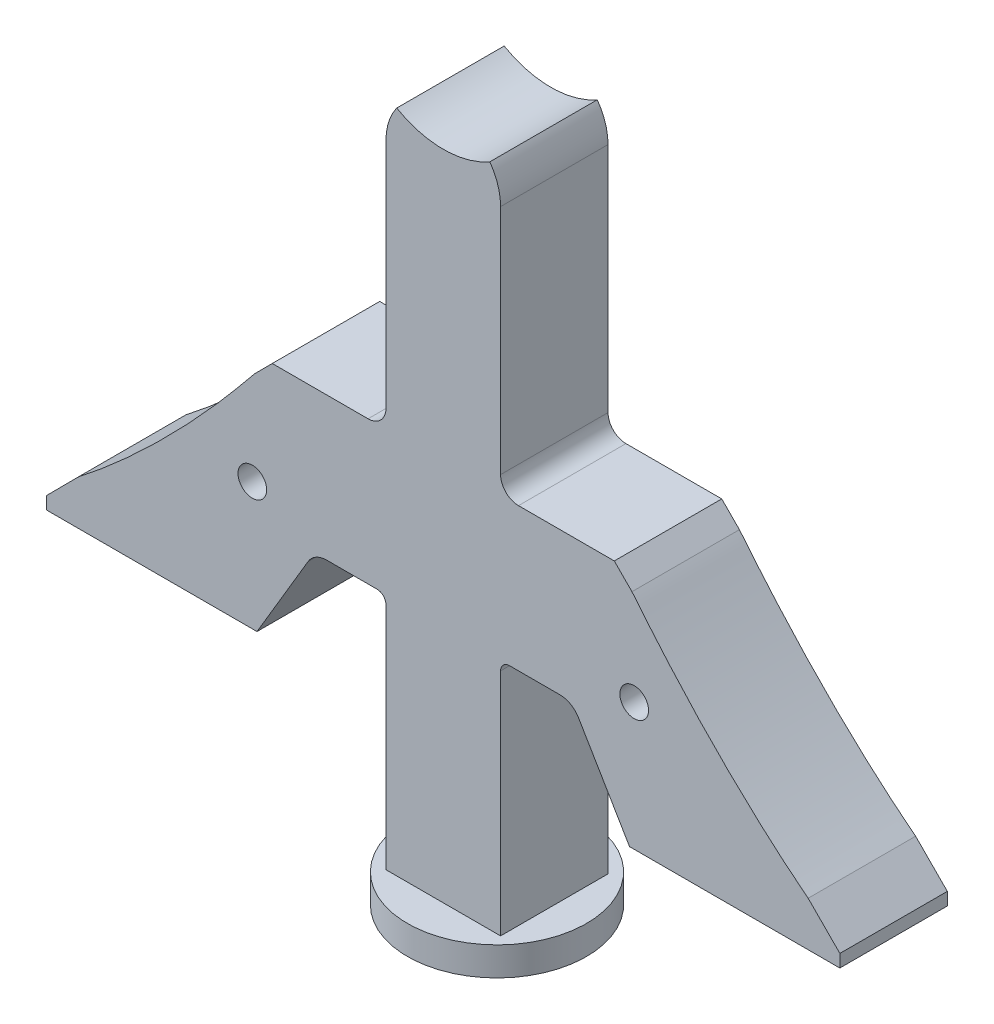
from build123d import *
from OCP.BRepFilletAPI import BRepFilletAPI_MakeChamfer

# Parameters (mm, degrees)
BOSS_EXTRUDE1_DEPTH      = 10
BOSS_EXTRUDE2_DEPTH      = 10
SKETCH72_R               = 5
CUT_EXTRUDE2_DEPTH       = 10
CUT_EXTRUDE4_DEPTH       = 14
CUT_EXTRUDE4_DEPTH_BACK  = 19
BOSS_EXTRUDE3_START      = 20
BOSS_EXTRUDE3_DEPTH      = 20
CUT_EXTRUDE5_DEPTH       = 19
CUT_EXTRUDE5_DEPTH_BACK  = 48
SKETCH146_R              = 5
CUT_EXTRUDE6_DEPTH       = 19
CUT_EXTRUDE6_DEPTH_BACK  = 19
CUT_EXTRUDE7_DEPTH       = 60
CUT_EXTRUDE8_DEPTH       = 72
CUT_EXTRUDE9_DEPTH       = 88
BOSS_EXTRUDE6_START      = -7.5
BOSS_EXTRUDE6_DEPTH      = 7.5
CUT_EXTRUDE10_DEPTH      = 19
CUT_EXTRUDE10_DEPTH_BACK = 41
SKETCH171_R              = 5
BOSS_EXTRUDE7_DEPTH      = 7.5
SKETCH172_W              = 3
SKETCH172_H              = 35.030253814
BOSS_EXTRUDE8_DEPTH      = 15
SKETCH173_W              = 32
SKETCH173_H              = 200
BOSS_EXTRUDE9_DEPTH      = 30
CHAMFER1_SIZE            = 5
CHAMFER1_SIZE2           = 3.535553346
FILLET1_R                = 5
CUT_EXTRUDE11_DEPTH      = 30
SKETCH175_W              = 47.76869264
SKETCH175_H              = 185.151923251
CUT_EXTRUDE12_DEPTH      = 55
SKETCH151_R              = 4
CUT_EXTRUDE14_DEPTH      = 15
SKETCH153_R              = 4
CUT_EXTRUDE15_DEPTH      = 15
CHAMFER3_SIZE            = 0.5
BOSS_EXTRUDE10_DEPTH     = 30
CUT_EXTRUDE16_DEPTH      = 181.457563316
SKETCH179_R              = 25
BOSS_EXTRUDE11_DEPTH     = 8


with BuildPart() as part:
    # Sketch1 → Boss-Extrude1 (new body)
    with BuildSketch(Plane.XY):
        with BuildLine():
            Line((-15, 37.030253814), (-15, -127.65801455))
            Line((-15, -127.65801455), (15, -127.65801455))
            Line((15, -127.65801455), (15, 37.030253814))
            ThreePointArc((15, 37.030253814), (0, 52.030253814), (-15, 37.030253814))
        make_face()
    extrude(amount=BOSS_EXTRUDE1_DEPTH)

    # Sketch2 → Boss-Extrude2 (add)
    with BuildSketch(Plane(origin=(0, 0, 0), x_dir=(-1, 0, 0), z_dir=(0, 0, -1))):
        Polygon((0, -15), (30.09, -15), (139.247111701, -124.883480474), (-139.247111701, -124.883480474), (-30.09, -15), align=None)
    extrude(amount=-BOSS_EXTRUDE2_DEPTH)

    # Sketch72 → Cut-Extrude2 (cut)
    with BuildSketch(Plane.XY.offset(10)):
        with Locations((0, 37.030253814)):
            Circle(SKETCH72_R)
    extrude(amount=-CUT_EXTRUDE2_DEPTH, mode=Mode.SUBTRACT)

    # Sketch144 → Cut-Extrude4 (cut, two sides: drawn at the far end of the back side and taken through both)
    with BuildSketch(Plane.XY.offset(10).offset(-CUT_EXTRUDE4_DEPTH_BACK)):
        with BuildLine():
            Line((-13, 37.030253814), (-13, -15))
            Line((-13, -15), (-23, -15))
            Line((-23, -15), (-23, 37.030253814))
            ThreePointArc((-23, 37.030253814), (0, 60.030253814), (23, 37.030253814))
            Line((23, 37.030253814), (23, -15))
            Line((23, -15), (13, -15))
            Line((13, -15), (13, 37.030253814))
            ThreePointArc((13, 37.030253814), (0, 50.030253814), (-13, 37.030253814))
        make_face()
    extrude(amount=CUT_EXTRUDE4_DEPTH + CUT_EXTRUDE4_DEPTH_BACK, mode=Mode.SUBTRACT)

    # Sketch145 → Boss-Extrude3 (add)
    with BuildSketch(Plane(origin=(0, 0, 0), x_dir=(-1, 0, 0), z_dir=(0, 0, -1)).offset(BOSS_EXTRUDE3_START)):
        with BuildLine():
            Line((30.09, -15), (13, -15))
            Line((13, -15), (13, 37.030253814))
            ThreePointArc((13, 37.030253814), (0, 50.030253814), (-13, 37.030253814))
            Line((-13, 37.030253814), (-13, -15))
            Line((-13, -15), (-30.09, -15))
            Line((-30.09, -15), (-139.247111701, -124.883480474))
            Line((-139.247111701, -124.883480474), (-15, -124.883480474))
            Line((-15, -124.883480474), (-15, -127.65801455))
            Line((-15, -127.65801455), (15, -127.65801455))
            Line((15, -127.65801455), (15, -124.883480474))
            Line((15, -124.883480474), (139.247111701, -124.883480474))
            Line((139.247111701, -124.883480474), (30.09, -15))
        make_face()
    extrude(amount=-BOSS_EXTRUDE3_DEPTH)

    # Sketch146 → Cut-Extrude5 (cut, two sides: drawn at the far end of the back side and taken through both)
    with BuildSketch(Plane.XY.offset(-CUT_EXTRUDE5_DEPTH_BACK)):
        with Locations((0, 37.030253814)):
            Circle(SKETCH146_R)
    extrude(amount=CUT_EXTRUDE5_DEPTH + CUT_EXTRUDE5_DEPTH_BACK, mode=Mode.SUBTRACT)

    # Sketch147 → Cut-Extrude6 (cut, two sides: drawn at the far end of the back side and taken through both)
    with BuildSketch(Plane(origin=(0, 0, 0), x_dir=(0, 0, -1), z_dir=(1, 0, 0)).offset(-CUT_EXTRUDE6_DEPTH_BACK)):
        Polygon((-2.5, 50.030253814), (-2.5, 20.030253814), (12.5, 20.030253814), (12.5, 50.030253814), (5, 50.030253814), align=None)
    extrude(amount=CUT_EXTRUDE6_DEPTH + CUT_EXTRUDE6_DEPTH_BACK, mode=Mode.SUBTRACT)

    # Sketch150 → Cut-Extrude7 (cut)
    with BuildSketch(Plane.XY.offset(10)):
        Polygon((-139.247111701, -124.883480474), (-114.247111701, -124.883480474), (-114.247111701, -93.838923463), (-155.604312259, -93.838923463), align=None)
        Polygon((139.247111701, -124.883480474), (114.247111701, -124.883480474), (114.247111701, -93.838923463), (144.778818184, -93.838923463), align=None)
    extrude(amount=-CUT_EXTRUDE7_DEPTH, mode=Mode.SUBTRACT)

    # Sketch155 → Cut-Extrude8 (cut)
    with BuildSketch(Plane(origin=(0, 0, -20), x_dir=(-1, 0, 0), z_dir=(0, 0, -1))):
        Polygon((-114.247111701, -99.71712192), (114.247111701, -99.71712192), (132.998124018, -127.280721413), (-4.838954003, -174.810748317), (-128.945135363, -139.691339549), align=None)
    extrude(amount=-CUT_EXTRUDE8_DEPTH, mode=Mode.SUBTRACT)

    # Sketch168 → Cut-Extrude9 (cut)
    with BuildSketch(Plane.XY.offset(10)):
        with BuildLine():
            Line((-102.627965354, -87.973722378), (-98.21134674, -23.838785425))
            Line((-98.21134674, -23.838785425), (-52.676683547, -37.736983068))
            add(Edge.make_bspline(
                [(-52.676683547, -37.736983068), (-53.448253243, -38.604940944), (-54.758018803, -40.255486938), (-56.393307349, -42.24544513), (-57.59393724, -43.693311358), (-58.490883563, -44.765164273), (-59.386563239, -45.826752691), (-60.281018922, -46.878039923), (-61.174144179, -47.919111167), (-62.065873359, -48.950018312), (-62.956131171, -49.970821146), (-63.844846057, -50.981576429), (-64.731946625, -51.982340808), (-65.617362588, -52.973170047), (-66.501024502, -53.954119244), (-67.382863834, -54.925242774), (-68.262812936, -55.886594308), (-69.140805058, -56.83822681), (-70.016774341, -57.78019253), (-70.890655834, -58.712543006), (-71.762385492, -59.635329052), (-72.6319002, -60.548600748), (-73.499137782, -61.452407427), (-74.36403703, -62.346797658), (-75.226537723, -63.231819226), (-76.086580666, -64.107519102), (-76.944107728, -64.97394342), (-77.799061885, -65.83113743), (-78.651387281, -66.679145464), (-79.501029286, -67.518010878), (-80.347934579, -68.347775997), (-81.192051232, -69.16848204), (-82.033328819, -69.980169042), (-82.871718537, -70.782875754), (-83.707173346, -71.576639531), (-84.539648144, -72.3614962), (-85.369099962, -73.137479905), (-86.195488195, -73.90462292), (-87.018774882, -74.662955436), (-87.838925031, -75.412505303), (-88.655907003, -76.153297726), (-89.469692983, -76.885354899), (-90.280259527, -77.608695576), (-91.08758824, -78.323334537), (-91.89166658, -79.029281964), (-92.692488851, -79.726542658), (-93.490057409, -80.415115104), (-94.284384181, -81.094990278), (-95.075492456, -81.766150286), (-95.86341948, -82.428566214), (-96.6482185, -83.08219705), (-97.429965937, -83.726982263), (-98.208753829, -84.362854554), (-98.984742254, -84.989673948), (-99.757998209, -85.607446121), (-100.529132919, -86.215484264), (-101.170253751, -86.716417382), (-101.895413536, -87.270801703), (-102.35237684, -87.641445426), (-102.627965354, -87.973722378)],
                knots=[0, 0, 0, 0, 0.049042517, 0.089027758, 0.108836127, 0.128522053, 0.148085836, 0.167527768, 0.186848129, 0.20604719, 0.225125215, 0.244082454, 0.262919153, 0.281635546, 0.30023186, 0.318708314, 0.337065118, 0.355302476, 0.373420583, 0.391419629, 0.409299796, 0.427061258, 0.444704186, 0.462228743, 0.479635086, 0.496923368, 0.514093738, 0.531146337, 0.548081305, 0.564898777, 0.581598887, 0.598181763, 0.614647534, 0.630996326, 0.647228265, 0.66334348, 0.679342097, 0.695224248, 0.710990068, 0.7266397, 0.742173292, 0.757591004, 0.772893008, 0.788079493, 0.803150668, 0.81810677, 0.832948063, 0.847674856, 0.862287502, 0.876786419, 0.8911721, 0.905445137, 0.919606246, 0.933656302, 0.94759639, 0.961427866, 0.975152458, 0.981975355, 1, 1, 1, 1], degree=3))
        make_face()
    cut_extrude9 = extrude(amount=-CUT_EXTRUDE9_DEPTH, mode=Mode.SUBTRACT)

    # Mirror1: Cut-Extrude9 across plane
    add(cut_extrude9.mirror(Plane(origin=(0, 0, 0), x_dir=(0, 0, 1), z_dir=(1, 0, 0))), mode=Mode.SUBTRACT)

    # Sketch169 → Boss-Extrude6 (add)
    with BuildSketch(Plane.XY.offset(10).offset(BOSS_EXTRUDE6_START)):
        with BuildLine():
            Line((-16, -15), (-13, -15))
            Line((-13, -15), (-13, 37.030253814))
            ThreePointArc((-13, 37.030253814), (-12.375631297, 41.010674647), (-10.5625, 44.608749295))
            Line((-10.5625, 44.608749295), (-16, 37.030253814))
            Line((-16, 37.030253814), (-16, -15))
        make_face()
        with BuildLine():
            Line((16, -15), (16, 37.030253814))
            Line((16, 37.030253814), (10.5625, 44.608749295))
            ThreePointArc((10.5625, 44.608749295), (12.375631297, 41.010674647), (13, 37.030253814))
            Line((13, 37.030253814), (13, -15))
            Line((13, -15), (16, -15))
        make_face()
    extrude(amount=BOSS_EXTRUDE6_DEPTH)

    # Sketch170 → Cut-Extrude10 (cut, two sides: drawn at the far end of the back side and taken through both)
    with BuildSketch(Plane.XY.offset(10).offset(-CUT_EXTRUDE10_DEPTH_BACK)):
        Polygon((-63.887492501, -32.771153319), (-27.188421499, -2.740818682), (-16, -2.740818682), (-16, -15), (-16, -32.771153319), align=None)
        Polygon((16, -15), (16, -32.771153319), (63.887492501, -32.771153319), (27.188421499, -2.740818682), (16, -2.740818682), align=None)
    extrude(amount=CUT_EXTRUDE10_DEPTH + CUT_EXTRUDE10_DEPTH_BACK, mode=Mode.SUBTRACT)

    # Sketch171 → Boss-Extrude7 (add)
    with BuildSketch(Plane(origin=(0, 0, -20), x_dir=(-1, 0, 0), z_dir=(0, 0, -1))):
        with BuildLine():
            Line((16, -15), (-16, -15))
            Line((-16, -15), (-16, 37.030253814))
            Line((-16, 37.030253814), (-10.5625, 44.608749295))
            ThreePointArc((-10.5625, 44.608749295), (0, 50.030253814), (10.5625, 44.608749295))
            Line((10.5625, 44.608749295), (16, 37.030253814))
            Line((16, 37.030253814), (16, -15))
        make_face()
        with Locations(Location((0, 37.030253814, 0), (0, 0, 180))):
            Circle(SKETCH171_R, mode=Mode.SUBTRACT)
    extrude(amount=-BOSS_EXTRUDE7_DEPTH)

    # Sketch172 → Boss-Extrude8 (add)
    with BuildSketch(Plane(origin=(0, 0, 2.5), x_dir=(-1, 0, 0), z_dir=(0, 0, -1))):
        with Locations((-14.5, 2.515126907)):
            Rectangle(SKETCH172_W, SKETCH172_H)
        with Locations((14.5, 2.515126907)):
            Rectangle(SKETCH172_W, SKETCH172_H)
    extrude(amount=BOSS_EXTRUDE8_DEPTH)

    # Sketch173 → Boss-Extrude9 (add)
    with BuildSketch(Plane(origin=(0, 0, -20), x_dir=(-1, 0, 0), z_dir=(0, 0, -1))):
        with Locations((0, -199.71712192)):
            Rectangle(SKETCH173_W, SKETCH173_H)
    extrude(amount=-BOSS_EXTRUDE9_DEPTH)

    # Chamfer1: one chamfer whose edges measure the first distance from different faces: ONE call of the kernel's chamfer builder (chamfer() names one face for all edges)
    chamfer1_edges_1 = [part.edges().sort_by_distance(p)[0] for p in [
        (-114.247111701, -99.71712192, -5),
    ]]
    chamfer1_side_1 = [part.faces().sort_by_distance(p)[0] for p in [
        (-108.057185848, -93.486006182, -5),
    ]]
    chamfer1_edges_2 = [part.edges().sort_by_distance(p)[0] for p in [
        (114.247111701, -99.71712192, -5),
    ]]
    chamfer1_side_2 = [part.faces().sort_by_distance(p)[0] for p in [
        (108.057185848, -93.486006182, -5),
    ]]
    chamfer1 = BRepFilletAPI_MakeChamfer(part.part.solid().wrapped)
    for e in chamfer1_edges_1:
        chamfer1.Add(CHAMFER1_SIZE, CHAMFER1_SIZE2, e.wrapped, chamfer1_side_1[0].wrapped)  # the first distance lies on this face
    for e in chamfer1_edges_2:
        chamfer1.Add(CHAMFER1_SIZE, CHAMFER1_SIZE2, e.wrapped, chamfer1_side_2[0].wrapped)  # the first distance lies on this face
    add(Compound.cast(chamfer1.Shape()), mode=Mode.REPLACE)

    # Fillet1
    fillet1_edges = [part.edges().sort_by_distance(p)[0] for p in [
        (-16, -32.771153319, -5),
        (16, -32.771153319, -5),
    ]]
    fillet(fillet1_edges, radius=FILLET1_R)

    # Sketch174 → Cut-Extrude11 (cut)
    with BuildSketch(Plane.XY.offset(10)):
        with BuildLine():
            Line((-16, -99.71712192), (-16, -75.21712192))
            ThreePointArc((-16, -75.21712192), (-16.732233047, -73.449354967), (-18.5, -72.71712192))
            Line((-18.5, -72.71712192), (-32.581175633, -72.71712192))
            ThreePointArc((-32.581175633, -72.71712192), (-35.551622901, -73.504018907), (-37.742924834, -75.658307578))
            Line((-37.742924834, -75.658307578), (-52, -99.71712192))
            Line((-52, -99.71712192), (-16, -99.71712192))
        make_face()
        with BuildLine():
            Line((16, -99.71712192), (52, -99.71712192))
            Line((52, -99.71712192), (37.742924834, -75.658307578))
            ThreePointArc((37.742924834, -75.658307578), (35.551622901, -73.504018907), (32.581175633, -72.71712192))
            Line((32.581175633, -72.71712192), (18.5, -72.71712192))
            ThreePointArc((18.5, -72.71712192), (16.732233047, -73.449354967), (16, -75.21712192))
            Line((16, -75.21712192), (16, -99.71712192))
        make_face()
    extrude(amount=-CUT_EXTRUDE11_DEPTH, mode=Mode.SUBTRACT)

    # Sketch175 → Cut-Extrude12 (cut)
    with BuildSketch(Plane.XY.offset(10)):
        with Locations((-3.11565368, -231.878790674)):
            Rectangle(SKETCH175_W, SKETCH175_H)
    extrude(amount=-CUT_EXTRUDE12_DEPTH, mode=Mode.SUBTRACT)

    # Sketch151 → Cut-Extrude14 (cut)
    with BuildSketch(Plane.XY.offset(10)):
        with Locations((-53.305086147, -64.131398819)):
            Circle(SKETCH151_R)
    extrude(amount=-CUT_EXTRUDE14_DEPTH, mode=Mode.SUBTRACT)

    # Sketch153 → Cut-Extrude15 (cut)
    with BuildSketch(Plane.XY.offset(10)):
        with Locations(Location((53.305086147, -64.131398819, 0), (0, 0, 180))):
            Circle(SKETCH153_R)
    extrude(amount=-CUT_EXTRUDE15_DEPTH, mode=Mode.SUBTRACT)

    # Chamfer3
    chamfer3_edges = [part.edges().sort_by_distance(p)[0] for p in [
        (-5, 37.030253814, 2.5),
        (0, 20.030253814, 2.5),
        (-13.28125, 40.819501555, 2.5),
        (-16, 28.530253814, 2.5),
        (0, 50.030253814, 2.5),
        (13.28125, 40.819501555, 2.5),
        (0, 50.030253814, -12.5),
        (13.28125, 40.819501555, -12.5),
        (-13.28125, 40.819501555, -12.5),
        (16, 28.530253814, 2.5),
        (16, 20.030253814, -5),
        (-16, 20.030253814, -5),
    ]]
    chamfer(chamfer3_edges, length=CHAMFER3_SIZE)

    # Sketch177 → Boss-Extrude10 (add)
    with BuildSketch(Plane.XY.offset(10)):
        with BuildLine():
            Line((-16, 37.030253814), (-16, -27.771153319))
            Line((-16, -27.771153319), (16, -27.771153319))
            Line((16, -27.771153319), (16, 37.030253814))
            ThreePointArc((16, 37.030253814), (0, 53.030253814), (-16, 37.030253814))
        make_face()
    extrude(amount=-BOSS_EXTRUDE10_DEPTH)

    # Sketch178 → Cut-Extrude16 (cut, through all)
    with BuildSketch(Plane.XY.offset(10)):
        with BuildLine():
            Line((0, 68.874293366), (-13, 46.357632868))
            ThreePointArc((-13, 46.357632868), (0, 42.874293366), (13, 46.357632868))
            Line((13, 46.357632868), (0, 68.874293366))
        make_face()
    extrude(amount=-CUT_EXTRUDE16_DEPTH, mode=Mode.SUBTRACT)

    # Sketch179 → Boss-Extrude11 (add)
    with BuildSketch(Plane.XZ.offset(139.302829048)):
        with Locations(Location((0, -5, 0), (0, 0, 270))):
            Circle(SKETCH179_R)
    extrude(amount=BOSS_EXTRUDE11_DEPTH)


solid = part.part
